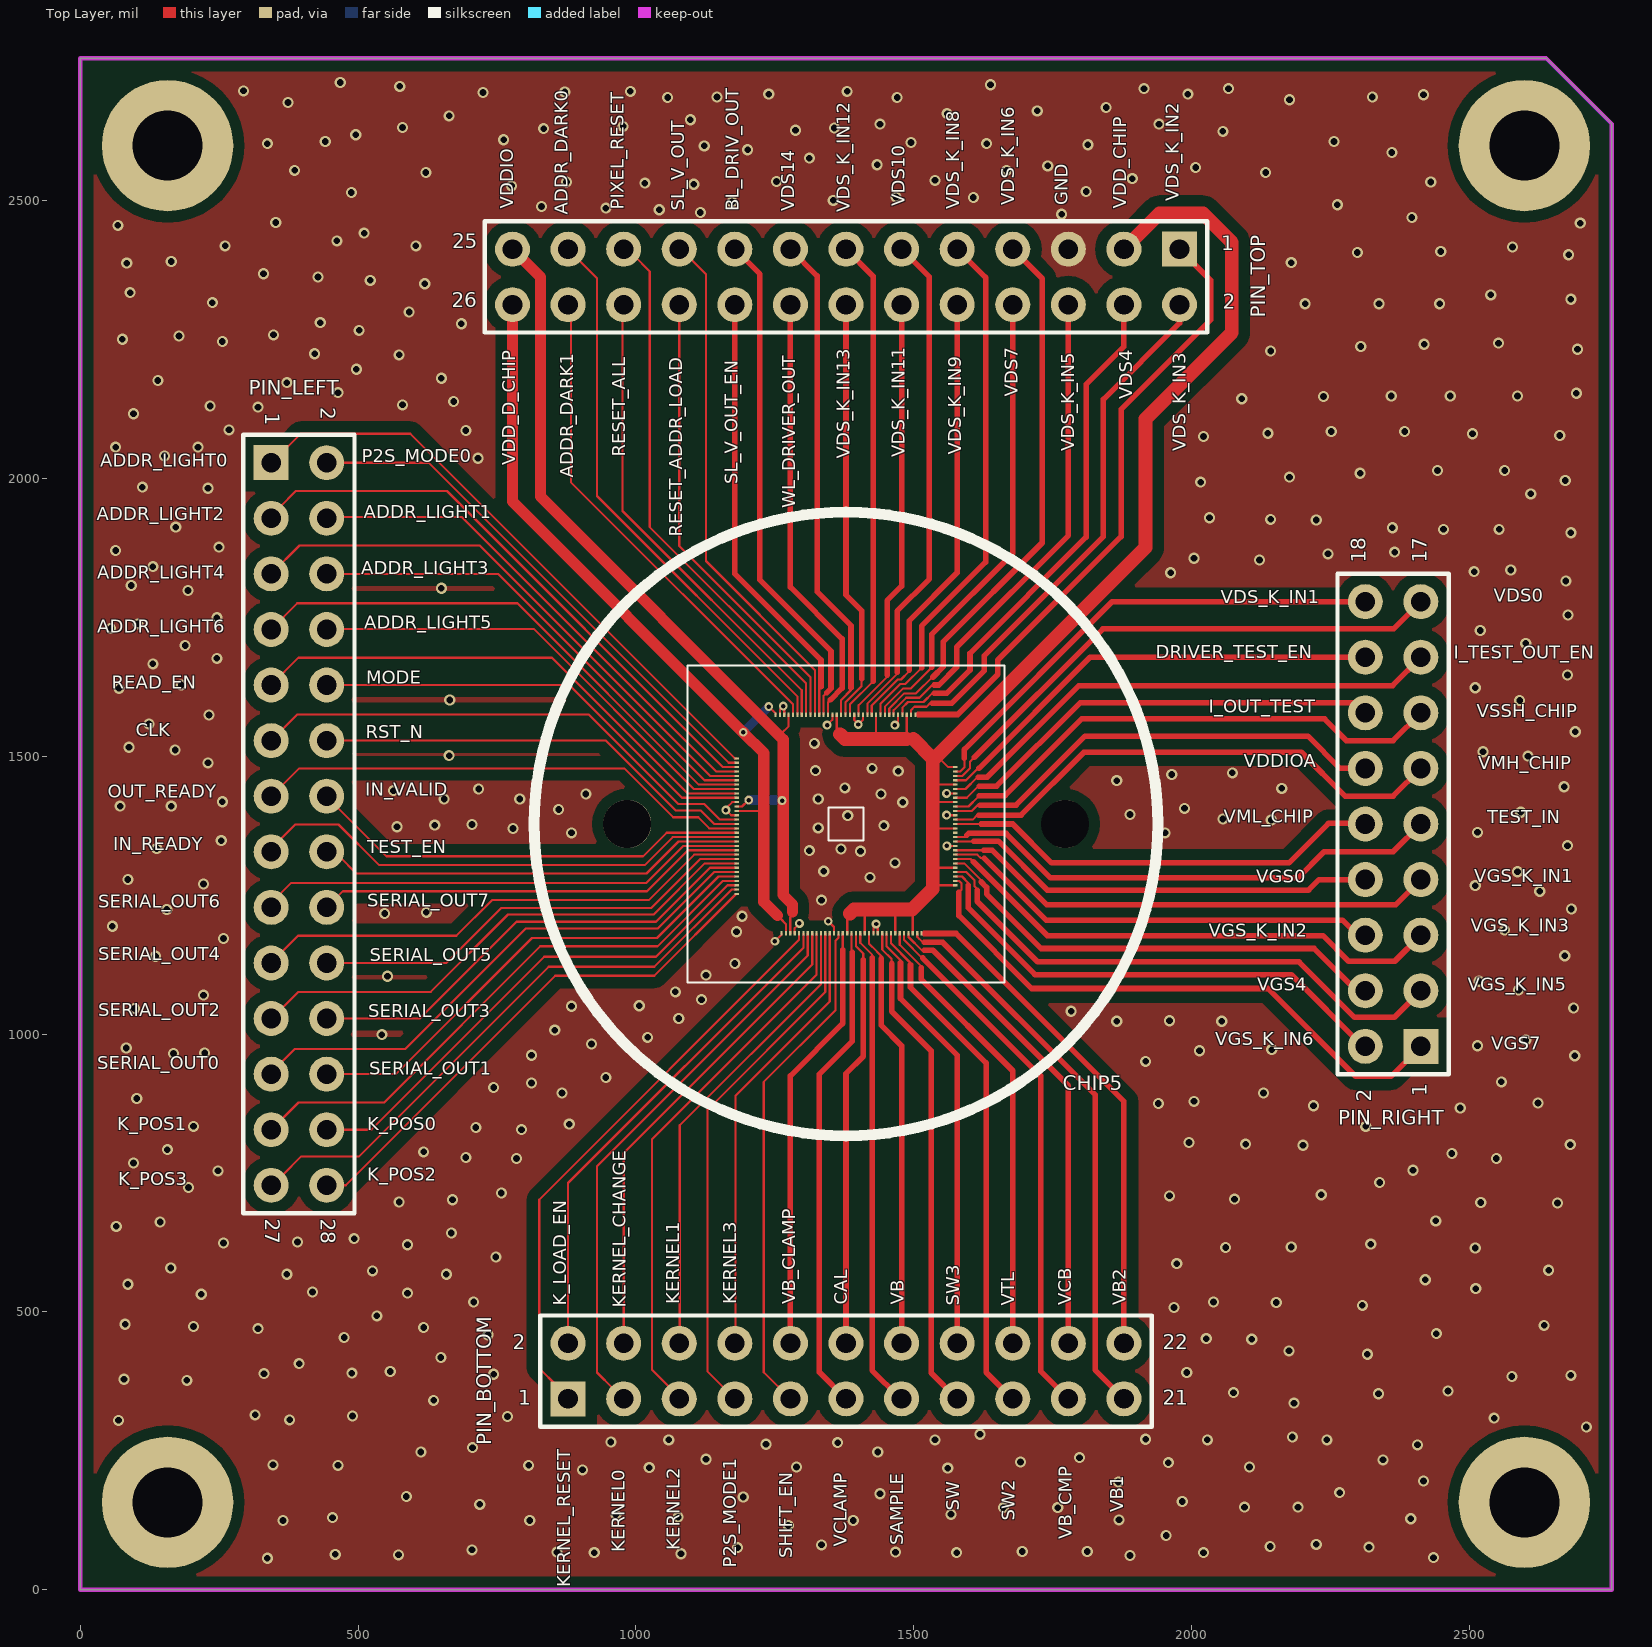
[diagram p0: Top Layer view]
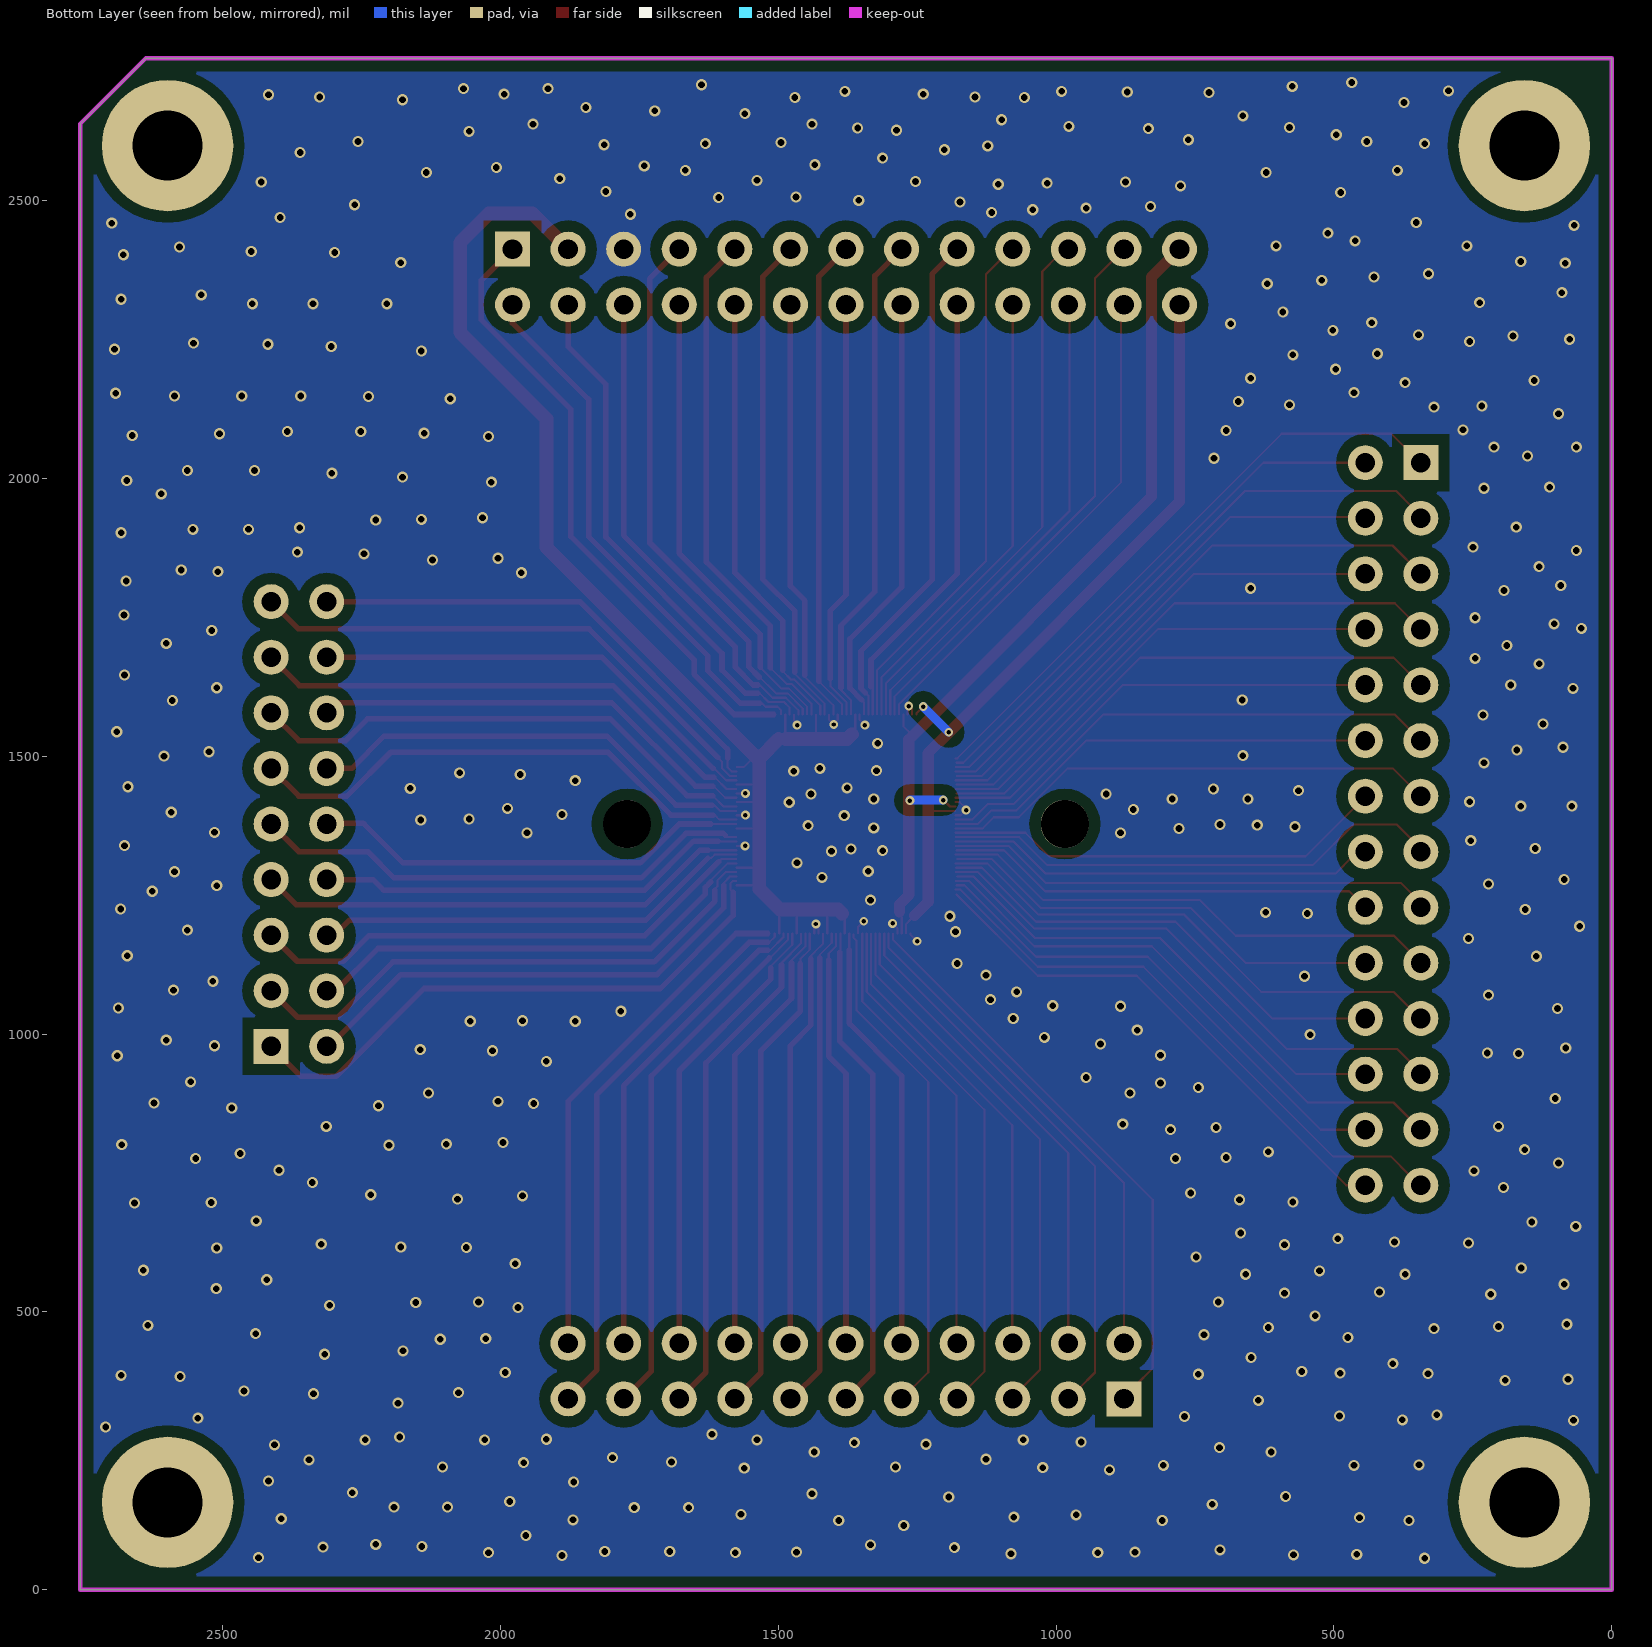
[diagram p1: Bottom Layer view, seen from below]
# Altium PCB MISC82784.pcbdoc
Units mil, origin at the board's own origin, x right, y up, seen from the top; angles counter-clockwise.
Board outline 2755.91 x 2755.91 mil, 2 copper layers (Top Layer, Bottom Layer); 5 components, 95 nets, 226 pads, 480 vias.

## Layer stack, top to bottom (the 12.6 mil dielectric is the usual default, probably not edited)
Top Layer: signal copper 1.4
Dielectric: dielectric 12.6, FR-4, Dk 4.8
Bottom Layer: signal copper 1.4

## Board outline
0,0 2755.91,0 2755.91,2637.4 2637.4,2755.91 0,2755.91

## Design rules (kind name [scope] priority, off if disabled: settings)
Clearance Clearance_2 [INPOLYGON] p1: gap=20
Clearance Clearance_1 [ispad vs ispad] p2: gap=3.9
Clearance [All] p3: gap=3.95
HoleSize [All] p1: absolutevalues=TRUE maxlimit=500 minlimit=1 maxpercent=80.000 minpercent=20.000
HoleToHoleClearance [All] p1: gap=0 allowstackedmicrovias=TRUE
MinimumSolderMaskSliver [All] p1: minsoldermaskwidth=0
PlaneConnect [All] p1: planeconnectstyle=Direct reliefexpansion=20 reliefentries=4 reliefconductorwidth=10 reliefairgap=10
PolygonConnect [All] p1: connectstyle=Direct reliefconductorwidth=10 reliefentries=4 polygonreliefangle="90 Angle"
RoutingVias [All] p1: holewidth=8 width=16 viastyle="Through Hole" minholewidth=8 minwidth=16 maxholewidth=12 maxwidth=20
SilkToSilkClearance [All] p1: silktosilkclearance=0
SilkscreenOverComponentPads [All] p1: minsilkscreentomaskgap=0
SolderMaskExpansion [All] p1: expansion=4
Width [All] p1: maxlimit=40 minlimit=3.9 preferedwidth=4 minimp=50.000000 maximp=50.000000 favimp=50.000000
22 further rules are at their usual default settings.

## Components (designator, comment, footprint, x,y, rotation, side; value= is the part's Value field where it differs from the comment)
CHIP5 "chip5" JSZ 1377.95,1377.95 r0 top locked
PIN_BOTTOM "#NAME?" HDR2.54-LI-2X11P 1377.95,393.7 r0 top
PIN_LEFT "#NAME?" HDR2.54-LI-2X14P 393.7,1377.95 r270 top
PIN_RIGHT "#NAME?" HDR2.54-LI-2X9P 2362.2,1377.95 r90 top
PIN_TOP "#NAME?" HDR2.54-LI-2X13P 1377.95,2362.2 r180 top

## Footprints (in the part's own frame and the unit in brackets; to place one, negate y for a bottom-side part, rotate by r counter-clockwise, add the part's x,y. Pads: shape width x height; smd on the part's side, far side on the other; paste and mask are expansions set on the pad)
HDR2.54-LI-2X9P [mm]
  rect 1.6x1.6 hole 0.9: 1(-10.16,-1.27)
  round 1.6 hole 0.9: 2(-10.16,1.27) 3(-7.62,-1.27) 4(-7.62,1.27) 5(-5.08,-1.27) 6(-5.08,1.27) 7(-2.54,-1.27) 8(-2.54,1.27) 9(0,-1.27) 10(0,1.27) 11(2.54,-1.27) 12(2.54,1.27) 13(5.08,-1.27) 14(5.08,1.27) 15(7.62,-1.27) 16(7.62,1.27) 17(10.16,-1.27) 18(10.16,1.27)
  silkscreen extent -11.43,-2.54 11.43,2.54
HDR2.54-LI-2X11P [mm]
  rect 1.6x1.6 hole 0.9: 1(-12.7,-1.27)
  round 1.6 hole 0.9: 2(-12.7,1.27) 3(-10.16,-1.27) 4(-10.16,1.27) 5(-7.62,-1.27) 6(-7.62,1.27) 7(-5.08,-1.27) 8(-5.08,1.27) 9(-2.54,-1.27) 10(-2.54,1.27) 11(0,-1.27) 12(0,1.27) 13(2.54,-1.27) 14(2.54,1.27) 15(5.08,-1.27) 16(5.08,1.27) 17(7.62,-1.27) 18(7.62,1.27) 19(10.16,-1.27) 20(10.16,1.27) 21(12.7,-1.27) 22(12.7,1.27)
  silkscreen extent -13.97,-2.54 13.97,2.54
HDR2.54-LI-2X13P [mm]
  rect 1.6x1.6 hole 0.9: 1(-15.24,-1.27)
  round 1.6 hole 0.9: 2(-15.24,1.27) 3(-12.7,-1.27) 4(-12.7,1.27) 5(-10.16,-1.27) 6(-10.16,1.27) 7(-7.62,-1.27) 8(-7.62,1.27) 9(-5.08,-1.27) 10(-5.08,1.27) 11(-2.54,-1.27) 12(-2.54,1.27) 13(0,-1.27) 14(0,1.27) 15(2.54,-1.27) 16(2.54,1.27) 17(5.08,-1.27) 18(5.08,1.27) 19(7.62,-1.27) 20(7.62,1.27) 21(10.16,-1.27) 22(10.16,1.27) 23(12.7,-1.27) 24(12.7,1.27) 25(15.24,-1.27) 26(15.24,1.27)
  silkscreen extent -16.51,-2.54 16.51,2.54
HDR2.54-LI-2X14P [mm]
  rect 1.6x1.6 hole 0.9: 1(-16.51,-1.27)
  round 1.6 hole 0.9: 2(-16.51,1.27) 3(-13.97,-1.27) 4(-13.97,1.27) 5(-11.43,-1.27) 6(-11.43,1.27) 7(-8.89,-1.27) 8(-8.89,1.27) 9(-6.35,-1.27) 10(-6.35,1.27) 11(-3.81,-1.27) 12(-3.81,1.27) 13(-1.27,-1.27) 14(-1.27,1.27) 15(1.27,-1.27) 16(1.27,1.27) 17(3.81,-1.27) 18(3.81,1.27) 19(6.35,-1.27) 20(6.35,1.27) 21(8.89,-1.27) 22(8.89,1.27) 23(11.43,-1.27) 24(11.43,1.27) 25(13.97,-1.27) 26(13.97,1.27) 27(16.51,-1.27) 28(16.51,1.27)
  silkscreen extent -17.78,-2.54 17.78,2.54
JSZ [mm]
  round 2.2 hole 2.2 unplated: 0(-10,0)
  oval 2x2.2 hole 2.2 unplated: 0(10,0)
  rect 0.1x0.2 smd: 1(3.177,5) 2(2.977,5) 3(2.777,5) 4(2.577,5) 5(2.377,5) 6(2.177,5) 7(1.977,5) 8(1.777,5) 9(1.577,5) 10(1.377,5) 11(1.177,5) 12(0.977,5) 13(0.777,5) 14(0.577,5) 15(0.377,5) 16(0.177,5) 17(-0.023,5) 18(-0.223,5) 19(-0.423,5) 20(-0.623,5) 21(-0.823,5) 22(-1.023,5) 23(-1.223,5) 24(-1.423,5) 25(-1.623,5) 26(-1.823,5) 27(-2.023,5) 28(-2.223,5) 29(-2.423,5) 30(-2.623,5) 31(-2.823,5) 32(-3.023,5) 33(-3.223,5) 66(-2.946,-5) 67(-2.746,-5) 68(-2.546,-5) 69(-2.346,-5) 70(-2.146,-5) 71(-1.946,-5) 72(-1.746,-5) 73(-1.546,-5) 74(-1.346,-5) 75(-1.146,-5) 76(-0.946,-5) 77(-0.746,-5) 78(-0.546,-5) 79(-0.346,-5) 80(-0.146,-5) 81(0.054,-5) 82(0.254,-5) 83(0.454,-5) 84(0.654,-5) 85(0.854,-5) 86(1.054,-5) 87(1.254,-5) 88(1.454,-5) 89(1.654,-5) 90(1.854,-5) 91(2.054,-5) 92(2.254,-5) 93(2.454,-5) 94(2.654,-5) 95(2.854,-5) 96(3.054,-5) 97(3.254,-5) 98(3.454,-5)
  rect 0.2x0.1 smd: 34(-5,3) 35(-5,2.8) 36(-5,2.6) 37(-5,2.4) 38(-5,2.2) 39(-5,2) 40(-5,1.8) 41(-5,1.6) 42(-5,1.4) 43(-5,1.2) 44(-5,1) 45(-5,0.8) 46(-5,0.6) 47(-5,0.4) 48(-5,0.2) 49(-5,0) 50(-5,-0.2) 51(-5,-0.4) 52(-5,-0.6) 53(-5,-0.8) 54(-5,-1) 55(-5,-1.2) 56(-5,-1.4) 57(-5,-1.6) 58(-5,-1.8) 59(-5,-2) 60(-5,-2.2) 61(-5,-2.4) 62(-5,-2.6) 63(-5,-2.8) 64(-5,-3) 65(-5,-3.2) 99(5,-2.8) 100(5,-2.6) 101(5,-2.4) 102(5,-2.2) 103(5,-2) 104(5,-1.8) 105(5,-1.6) 106(5,-1.4) 107(5,-1.2) 108(5,-1) 109(5,-0.8) 110(5,-0.6) 111(5,-0.4) 112(5,-0.2) 113(5,0) 114(5,0.2) 115(5,0.4) 116(5,0.6) 117(5,0.8) 118(5,1) 119(5,1.2) 120(5,1.4) 121(5,1.6) 122(5,1.8) 123(5,2) 124(5,2.2) 125(5,2.4) 126(5,2.6)
  silkscreen extent -14.25,-14.25 14.25,14.25

## Part data
PIN_BOTTOM: library part PZ254-2-11-Z-8.5
PIN_LEFT: library part PZ254-2-14-Z-8.5
PIN_RIGHT: library part PZ254-2-09-Z-8.5
PIN_TOP: library part PZ254-2-13-Z-2.5-G1

## Free pads (board coordinates)
  round 236.22 hole 125.98: 0(157.48,157.48) 0(157.48,2598.43) 0(2598.43,157.48) 0(2598.43,2598.43)

## Via types
v1: diameter 20, hole 12, Top Layer to Bottom Layer, 464 vias
v2: diameter 16, hole 8, Top Layer to Bottom Layer, 16 vias

## Nets (pads, with @x,y where several pads share a name; then routed paths per layer and width w, separated by ;. In a path a pad name is that pad's centre, name@x,y a point inside that pad or via, vN(x,y) a via of type N, cw(c..) or ccw(c..) an arc to the next point about the centre after c; other vN are vias at no path point)
ADDR_DARK0: CHIP5.28 PIN_TOP.23 | length 984
  Top Layer w3.9: PIN_TOP.23@895,2395 930,2360 930,1968 1290.44,1607.56 CHIP5.28
ADDR_DARK1: CHIP5.29 PIN_TOP.24 | length 897.9
  Top Layer w3.9: PIN_TOP.24@877,2297 886,2297 883,2294 883,1993 1282.56,1593.44 CHIP5.29
ADDR_LIGHT0: CHIP5.34 PIN_LEFT.1 | length 1061.3
  Top Layer w3.9: PIN_LEFT.1@372,2055 397,2080 594,2080 1177.94,1496.06 CHIP5.34
ADDR_LIGHT1: CHIP5.37 PIN_LEFT.4 | length 898.6
  Top Layer w3.9: PIN_LEFT.4@472,1930 687,1930 1144.56,1472.44 CHIP5.37
ADDR_LIGHT2: CHIP5.36 PIN_LEFT.3 | length 1039.8
  Top Layer w3.9: PIN_LEFT.3@359,1948 388,1977 660,1977 1156.69,1480.31 CHIP5.36
ADDR_LIGHT3: CHIP5.39 PIN_LEFT.6 | length 878.9
  Top Layer w3.9: PIN_LEFT.6@456,1828 752,1828 1123.31,1456.69 CHIP5.39
ADDR_LIGHT4: CHIP5.38 PIN_LEFT.5 | length 1028.1
  Top Layer w3.9: PIN_LEFT.5 394.75,1879 719,1879 1133.43,1464.57 CHIP5.38@1179,1464.57
ADDR_LIGHT5: CHIP5.41 PIN_LEFT.8 | length 839.4
  Top Layer w3.9: PIN_LEFT.8@461,1729 816,1729 1104.06,1440.94 CHIP5.41
ADDR_LIGHT6: CHIP5.40 PIN_LEFT.7 | length 989.9
  Top Layer w3.9: PIN_LEFT.7 390.75,1775 787,1775 1113.18,1448.82 CHIP5.40@1179,1448.82
AOUT1: CHIP5.111
BL_DRIVER_OUT: CHIP5.22 PIN_TOP.17 | length 913.2
  Top Layer w3.9: CHIP5.22 1337.68,1608.68 1342,1613
  Top Layer w10: PIN_TOP.17 1223,2367.16 1223,1817 1351,1689 1351,1622 1343,1614
CAL: CHIP5.83 PIN_BOTTOM.12 | length 755.7
  Top Layer w3.9: CHIP5.83 1395.83,1158.17 1409,1145 1409,1134
  Top Layer w10: PIN_BOTTOM.12 1377.95,928.95 1409,960 1409,1134
CLK: CHIP5.48 PIN_LEFT.11 | length 935.2
  Top Layer w3.9: PIN_LEFT.11 390.75,1575 915,1575 1076,1414 1123,1414 1151.17,1385.83 CHIP5.48
DRIVER_TEST_EN: CHIP5.123 PIN_RIGHT.16 | length 825.6
  Top Layer w3.9: CHIP5.123 1593.69,1456.69 1614,1477
  Top Layer w10: 1617,1478 1816.95,1677.95 1886,1677.95 PIN_RIGHT.16
GND: CHIP5.5 CHIP5.13 CHIP5.15 CHIP5.20 CHIP5.31 CHIP5.32 CHIP5.44 CHIP5.47 CHIP5.66 CHIP5.69 CHIP5.78 CHIP5.87 CHIP5.88 CHIP5.108 CHIP5.115 CHIP5.120 PIN_TOP.5 | length 299.4
  Top Layer w3.9: v2(1162,1403) 1171.3,1393.7 CHIP5.47 ; v2@1163,1407 1173.32,1417.32 CHIP5.44 ; v2(1250,1167) 1261.97,1178.97 CHIP5.66 ; CHIP5.32 1258.94,1583.94 v2(1265,1590) ; CHIP5.31 v2@1266.82,1585.82 ; CHIP5.69 1285.59,1190.59 v2(1294,1199) ; v2(1344,1556) 1353.43,1565.43 CHIP5.20 ; v2(1346,1203) 1356.46,1192.54 CHIP5.78 ; CHIP5.15 1392.8,1565.2 v2@1398,1560 ; v2(1400,1557) 1408.55,1565.55 CHIP5.13 ; CHIP5.87 1427.32,1193.32 v2(1432,1198) ; CHIP5.88 v2@1435.2,1190.8 ; v2(1466,1556) 1471.54,1561.54 CHIP5.5 ; v2(1559,1394) 1559.3,1393.7 CHIP5.115 ; v2(1559.07,1433.07) CHIP5.120 ; v2(1559.42,1338.58) CHIP5.108
  Bottom Layer w3.9: v2@1249,1167 v2(1250,1167)
  other v1: 337,57 2435,58 1889,62 573,63 459,64 1081,65 925,67 1577,67 2021,67 858,68 1467,68 1695,69 1812,69 705,72 1183,76 2319,77 2141,78 1334,81 2224,82 1954,98 1274,116 365,125 809,125 1391,125 1869,126 2394,128 454,130 1076,131 964,135 1567,136 1661,148 1759,148 2095,149 2191,149 719,154 1983,159 1193,167 587,168 1439,173 2266,175 1868,194 2417,196 904,216 1561,219 1024,220 1289,221 2104,221 464,224 807,224 347,225 1958,229 1692,230 2344,234 1126,235 1798,238 613,248 1435,248 706,256 2406,261 1234,262 1363,265 955,266 1059,270 1538,270 2028,270 2243,270 1917,271 2181,275 1619,280 2710,293 69,305 377,306 2544,309 769,312 490,313 315,315 2184,336 636,341 2336,353 2075,355 2461,358 192,377 79,379 2576,384 2682,386 744,388 331,389 489,390 1991,391 558,393 394,407 649,418 2316,424 2175,430 2108,451 2026,452 475,454 734,459 2440,461 320,470 618,472 204,474 2634,476 81,478 534,493 1968,508 2307,512 2152,517 708,518 2039,518 218,532 589,534 418,536 2511,542 86,550 2420,558 372,568 659,568 526,574 2642,575 163,579 1973,587 748,599 2510,615 2061,616 2179,617 589,621 2322,622 258,624 391,626 493,632 668,642 65,654 144,662 2439,664 2658,696 2520,697 574,698 670,702 2077,703 1960,709 2233,711 758,714 195,724 2338,733 248,754 2398,755 96,768 785,776 2548,776 694,778 2468,785 618,788 157,792 2200,800 2681,801 2097,802 1995,805 794,828 712,832 204,834 2313,834 880,838 2483,867 2219,871 1940,875 2623,876 2004,879 102,884 867,894 2129,894 744,904 812,912 2557,914 946,922 1917,951 2689,961 812,962 168,965 224,966 2014,970 2144,972 83,975 2514,979 920,982 2601,989 1021,994 543,999 854,1007 1865,1023 2054,1023 1960,1024 1077,1028 1783,1041 98,1046 2687,1047 884,1050 1006,1051 1118,1062 222,1070 1071,1076 2588,1079 2517,1095 553,1104 1126,1106 1178,1127 136,1140 2671,1141 258,1172 1181,1184 2563,1187 58,1194 1191,1212 548,1217 623,1219 156,1224 2683,1225 1334,1241 2626,1257 2510,1267 222,1270 86,1278 1421,1282 2586,1292 1338,1293 1466,1308 1404,1329 1312,1330 1369,1333 138,1334 2676,1339 254,1348 884,1362 1952,1362 2514,1363 779,1370 1328,1371 570,1373 1446,1375 638,1376 705,1377 2143,1385 2056,1387 1381,1393 1889,1395 2592,1399 861,1404 1987,1406 72,1410 164,1410 1480,1417 256,1418 655,1423 791,1423 1328,1423 910,1432 1441,1432 564,1438 717,1441 2162,1442 1376,1443 2670,1445 1865,1456 1964,1467 2073,1470 1472,1473 1323,1474 1425,1478 230,1488 2605,1500 664,1501 2524,1508 171,1511 88,1516 1321,1523 2690,1544 124,1558 232,1574 2590,1600 665,1601 70,1622 2510,1623 182,1628 2676,1646 131,1666 246,1676 189,1699 2601,1703 2519,1726 55,1730 104,1738 246,1749 2677,1754 194,1798 650,1802 92,1807 2673,1815 1962,1830 2508,1832 2574,1835 131,1841 2122,1853 2004,1856 2245,1864 2365,1867 64,1870 250,1876 2682,1902 2453,1908 2553,1908 2361,1911 172,1912 2224,1925 2142,1926 2032,1929 2610,1972 230,1982 112,1984 2016,1993 2672,1996 2176,2002 2303,2009 2442,2014 2563,2014 716,2036 152,2040 64,2056 212,2056 2021,2075 2662,2077 2505,2080 2137,2081 2251,2084 2383,2084 694,2086 268,2087 96,2116 320,2128 234,2130 580,2132 672,2138 2090,2143 2237,2147 2359,2148 2465,2148 2586,2148 2692,2153 464,2154 372,2172 140,2176 650,2180 497,2196 574,2222 422,2224 2142,2229 2694,2232 2304,2237 2418,2241 2552,2243 256,2246 76,2250 178,2256 348,2258 502,2266 686,2278 432,2280 592,2299 2204,2314 2337,2314 2446,2314 238,2316 2682,2322 2538,2330 90,2334 620,2350 522,2356 428,2362 330,2368 84,2387 2179,2388 164,2390 2678,2402 2298,2406 2448,2408 2577,2416 261,2418 604,2418 462,2427 511,2441 68,2455 2699,2459 352,2460 2396,2469 1766,2475 1116,2478 1042,2483 946,2486 830,2489 2262,2492 1173,2497 1355,2500 1607,2505 1468,2506 488,2514 1810,2516 776,2526 1104,2529 1016,2531 875,2533 2430,2533 1253,2534 1538,2536 1893,2539 622,2550 2133,2550 386,2554 1667,2554 2007,2559 1741,2562 1434,2564 1312,2576 2360,2586 1201,2591 1123,2598 1813,2600 337,2602 1631,2602 1495,2604 441,2606 2256,2606 762,2609 496,2618 2056,2624 1287,2626 834,2629 1357,2630 580,2631 977,2633 1439,2637 1941,2637 1098,2645 664,2652 1560,2656 1722,2661 1846,2667 374,2676 2176,2681 1057,2685 1470,2685 1146,2686 2325,2686 2417,2690 1239,2691 1993,2691 725,2694 872,2695 990,2696 1380,2696 294,2697 1914,2701 2066,2701 575,2705 1638,2708 468,2712
I_OUT_TEST: CHIP5.119 PIN_RIGHT.14 | length 813.6
  Top Layer w3.9: CHIP5.119 1595.2,1425.2 1616,1446
  Top Layer w10: 1618,1446 1649,1446 1799,1596 2294.16,1596 PIN_RIGHT.14
I_TEST_OUT_EN: CHIP5.121 PIN_RIGHT.15 | length 932.2
  Top Layer w3.9: CHIP5.121 1592.94,1440.94 1613,1461
  Top Layer w10: 1616,1462 1632,1462 1797,1627 1810,1627 2361.25,1627 PIN_RIGHT.15
IN_READY: CHIP5.52 PIN_LEFT.15 | length 901.8
  Top Layer w3.9: PIN_LEFT.15@347,1337 387,1377 465,1377 538,1304 1016,1304 1066.33,1354.33 CHIP5.52
IN_VALID: CHIP5.51 PIN_LEFT.14 | length 789
  Top Layer w3.9: PIN_LEFT.14@451,1420 551,1320 1013,1320 1055.2,1362.2 CHIP5.51
K_LOAD_EN: CHIP5.71 PIN_BOTTOM.2 | length 912.8
  Top Layer w3.9: PIN_BOTTOM.2 877.95,731.95 1301.34,1155.34 CHIP5.71
K_POS0: CHIP5.63 PIN_LEFT.26 | length 917.5
  Top Layer w3.9: PIN_LEFT.26 523.95,827.95 835,1139 1036,1139 1164.71,1267.71 CHIP5.63@1179,1267.71
K_POS1: CHIP5.62 PIN_LEFT.25 | length 1004.1
  Top Layer w3.9: PIN_LEFT.25@357,841 393,877 547,877 828,1158 1039,1158 1156.59,1275.59 CHIP5.62
K_POS2: CHIP5.65 PIN_LEFT.28 | length 952
  Top Layer w3.9: PIN_LEFT.28 477.95,727.95 855,1105 1033,1105 CHIP5.65@1179,1251
K_POS3: CHIP5.64 PIN_LEFT.27 | length 1029.9
  Top Layer w3.9: PIN_LEFT.27@364,746 398,780 502,780 843,1121 1033,1121 1171.84,1259.84 CHIP5.64
KERNEL0: CHIP5.72 PIN_BOTTOM.3 | length 988.2
  Top Layer w3.9: PIN_BOTTOM.3@959,362 930,391 930,762 1309.21,1141.21 CHIP5.72
KERNEL1: CHIP5.75 PIN_BOTTOM.6 | length 827.2
  Top Layer w3.9: PIN_BOTTOM.6@1079,459 1079,836 1332.83,1089.83 CHIP5.75
KERNEL2: CHIP5.74 PIN_BOTTOM.5 | length 962.8
  Top Layer w3.9: PIN_BOTTOM.5@1068,357 1029,396 1029,811 1324.96,1106.96 CHIP5.74
KERNEL3: CHIP5.77 PIN_BOTTOM.8 | length 789.3
  Top Layer w3.9: PIN_BOTTOM.8@1179,462 1179,889 1348.58,1058.58 CHIP5.77
KERNEL_CHANGE: CHIP5.73 PIN_BOTTOM.4 | length 877.9
  Top Layer w3.9: PIN_BOTTOM.4 977.95,785.95 1317.09,1125.09 CHIP5.73
KERNEL_RESET: CHIP5.70 PIN_BOTTOM.1 | length 1021
  Top Layer w3.9: PIN_BOTTOM.1@858,367 826,399 826,702 1293.46,1169.46 CHIP5.70
MODE: CHIP5.43 PIN_LEFT.10 | length 809.1
  Top Layer w3.9: PIN_LEFT.10@456,1628 880,1628 1082.8,1425.2 CHIP5.43
OUT_READY: CHIP5.50 PIN_LEFT.13 | length 879.9
  Top Layer w3.9: PIN_LEFT.13@360,1444 394,1478 979,1478 1067,1390 1112,1390 1131.92,1370.08 CHIP5.50
P2S_MODE0: CHIP5.35 PIN_LEFT.2 | length 958.9
  Top Layer w3.9: PIN_LEFT.2 627.05,2027.95 1166.81,1488.19 CHIP5.35@1179,1488.19
P2S_MODE1: CHIP5.76 PIN_BOTTOM.7 | length 945.4
  Top Layer w3.9: PIN_BOTTOM.7 1129,392.65 1129,864 1340.71,1075.71 CHIP5.76
PIXEL_RESET_EN: CHIP5.26 PIN_TOP.21 | length 956.1
  Top Layer w3.9: PIN_TOP.21@995,2402 1025,2372 1025,1912 1306.19,1630.81 CHIP5.26
READ_EN: CHIP5.42 PIN_LEFT.9 | length 956.7
  Top Layer w3.9: PIN_LEFT.9 392.75,1677 849,1677 1092.92,1433.08 CHIP5.42@1179,1433.08
RESET_ADDR_LOAD: CHIP5.25 PIN_TOP.20 | length 835.2
  Top Layer w3.9: PIN_TOP.20@1077.95,2311 PIN_TOP.20 ; PIN_TOP.20@1078,2311 1078,1878 1314.06,1641.94 CHIP5.25
RESET_ALL: CHIP5.27 PIN_TOP.22 | length 870.9
  Top Layer w3.9: PIN_TOP.22@976,2301 976,1941 1298.31,1618.69 CHIP5.27 ; PIN_TOP.22@977.95,2301 PIN_TOP.22
RST_N: CHIP5.49 PIN_LEFT.12 | length 799.5
  Top Layer w3.9: PIN_LEFT.12 946.05,1527.95 1072,1402 1117,1402 1141.05,1377.95 CHIP5.49
SAMPLE: CHIP5.84 PIN_BOTTOM.13 | length 868.6
  Top Layer w3.9: CHIP5.84 1403.7,1164.3 1425,1143 1425,1137
  Top Layer w10: 1425,1137 1425,395 PIN_BOTTOM.13@1473,347 ; PIN_BOTTOM.13@1473.83,347.83 PIN_BOTTOM.13
SERIAL_OUT0: CHIP5.60 PIN_LEFT.23 | length 966.6
  Top Layer w3.9: PIN_LEFT.23@358,945 386,973 585,973 802,1190 1039,1190 1140.34,1291.34 CHIP5.60
SERIAL_OUT1: CHIP5.61 PIN_LEFT.24 | length 881.6
  Top Layer w3.9: PIN_LEFT.24 567.95,927.95 813,1173 1038,1173 1148.47,1283.47 CHIP5.61@1178,1283.47
SERIAL_OUT2: CHIP5.58 PIN_LEFT.21 | length 934.7
  Top Layer w3.9: PIN_LEFT.21@357,1040 393,1076 631,1076 770,1215 1032,1215 1124.09,1307.09 CHIP5.58
SERIAL_OUT3: CHIP5.59 PIN_LEFT.22 | length 848.7
  Top Layer w3.9: PIN_LEFT.22 610.95,1027.95 785,1202 1036,1202 1133.21,1299.21 CHIP5.59@1180,1299.21
SERIAL_OUT4: CHIP5.56 PIN_LEFT.19 | length 894.8
  Top Layer w3.9: PIN_LEFT.19@360,1145 392,1177 677,1177 741,1241 1023,1241 1104.83,1322.83 CHIP5.56
SERIAL_OUT5: CHIP5.57 PIN_LEFT.20 | length 811.8
  Top Layer w3.9: PIN_LEFT.20 658.95,1127.95 758,1227 1028,1227 1115.97,1314.97 CHIP5.57@1178,1314.97
SERIAL_OUT6: CHIP5.54 PIN_LEFT.17 | length 865.5
  Top Layer w3.9: PIN_LEFT.17@354,1246 380,1272 1019,1272 1085.58,1338.58 CHIP5.54
SERIAL_OUT7: CHIP5.55 PIN_LEFT.18 | length 777.9
  Top Layer w3.9: PIN_LEFT.18 472.75,1257 1020,1257 1093.71,1330.71 CHIP5.55@1179,1330.71
SHIFT_EN: CHIP5.79 PIN_BOTTOM.9 | length 910.8
  Top Layer w3.9: PIN_BOTTOM.9 1230,391.65 1230,914 1359,1043 1359,1168 1364.34,1173.34 CHIP5.79@1364.34,1179
SL_V_OUT: CHIP5.24 PIN_TOP.19 | length 918.6
  Top Layer w3.9: PIN_TOP.19@1094,2399 1126,2367 1126,1851 1321.94,1655.06 CHIP5.24
SL_V_OUT_EN: CHIP5.23 PIN_TOP.18 | length 803
  Top Layer w3.9: CHIP5.23 1329.81,1621.81 1333,1625
  Top Layer w10: PIN_TOP.18 1177.95,1828.05 1333,1673 1333,1625.16 1332.84,1625
SW: CHIP5.89 PIN_BOTTOM.15 | length 893.3
  Top Layer w3.9: CHIP5.89 1443.07,1151.93 1460,1135 1460,1127
  Top Layer w10: 1460,1127 1460,1041 1531,970 1531,390.65 PIN_BOTTOM.15
SW2: CHIP5.91 PIN_BOTTOM.17 | length 928.2
  Top Layer w3.9: CHIP5.91 1458.82,1163.18 1494,1128 1494,1125
  Top Layer w10: 1494,1125 1494,1084 1630,948 1630,391.65 PIN_BOTTOM.17
SW3: CHIP5.90 PIN_BOTTOM.16 | length 790.4
  Top Layer w3.9: CHIP5.90 1450.94,1168 1450.94,1166.06 1450.94,1158.06 1477,1132 1477,1128
  Top Layer w10: 1476,1128 1476,1064 1577.95,962.05 PIN_BOTTOM.16
TEST_EN: CHIP5.53 PIN_LEFT.16 | length 751.7
  Top Layer w3.9: PIN_LEFT.16@466,1320 497,1289 1019,1289 1076.46,1346.46 CHIP5.53
TEST_IN: CHIP5.110 PIN_RIGHT.9 | length 913.9
  Top Layer w3.9: CHIP5.110 1593.33,1354.33 1595.68,1356.68
  Top Layer w10: 1595,1357.36 1598.64,1361 1608,1361 1666,1361 1746,1281 2191,1281 2238,1328 2362.25,1328 PIN_RIGHT.9
VB: CHIP5.86 PIN_BOTTOM.14 | length 761.6
  Top Layer w3.9: CHIP5.86 1419.45,1162.55 1434,1148 1436,1146 1441,1141 1441,1136
  Top Layer w10: 1441,1136 1441,1016 1477.95,979.05 PIN_BOTTOM.14
VB1: CHIP5.97 PIN_BOTTOM.21 | length 1012.7
  Top Layer w3.9: CHIP5.97 1506.06,1174.73 1509.52,1171.27 1509.73,1171.27 1516,1165 1519,1165
  Top Layer w10: 1519,1165 1552,1165 1826,891 1826,395.65 PIN_BOTTOM.21
VB2: CHIP5.98 PIN_BOTTOM.22 | length 919.4
  Top Layer w10: 1519,1181 1576,1181 1877.95,879.05 PIN_BOTTOM.22
VB_CLAMP: CHIP5.80 PIN_BOTTOM.10 | length 776.4
  Top Layer w3.9: 1372.2,1152 CHIP5.80
  Top Layer w10: PIN_BOTTOM.10 1277.95,924.95 1372,1019 1372,1152
VB_CMP: CHIP5.94 PIN_BOTTOM.19 | length 960
  Top Layer w3.9: CHIP5.94 1482.44,1169.56 1515.31,1136.69
  Top Layer w10: 1515.68,1137.05 1728,924.73 1728,393.65 PIN_BOTTOM.19
VCB: CHIP5.95 PIN_BOTTOM.20 | length 868.3
  Top Layer w3.9: CHIP5.95 1490.31,1174.69 1514,1151 1519,1151
  Top Layer w10: 1519,1151 1534,1151 1777.95,907.05 PIN_BOTTOM.20
VCLAMP: CHIP5.82 PIN_BOTTOM.11 | length 879.7
  Top Layer w3.9: 1387.95,1149.05 CHIP5.82
  Top Layer w10: PIN_BOTTOM.11 1330,391.65 1330,928 1389,987 1389,1147
VDD_CHIP: CHIP5.3 CHIP5.10 CHIP5.19 CHIP5.81 CHIP5.85 CHIP5.92 CHIP5.96 CHIP5.99 CHIP5.103 CHIP5.112 CHIP5.118 CHIP5.122 CHIP5.126 PIN_TOP.3 | length 2461.6
  Top Layer w3.9: CHIP5.19 1361.31,1548.69 1369,1541 ; CHIP5.81 1380.08,1216.08 ; CHIP5.85 1411.57,1213.57 ; 1432.17,1531 CHIP5.10 ; CHIP5.92 1466.69,1215.69 ; 1487.29,1531 CHIP5.3 ; 1491,1224 1498.19,1216.81 CHIP5.96 ; 1534,1299.21 CHIP5.103 ; 1534,1417.32 CHIP5.118 ; 1534,1448.82 CHIP5.122 ; 1536,1267.72 CHIP5.99 ; 1537,1370.08 CHIP5.112 ; 1550,1492 1561.69,1480.31 CHIP5.126
  Top Layer w25: 1367.5,1539.5 1376,1531 1432.17,1531 1487.29,1531 ; 1385,1217 1392,1224 1491,1224 ; 1497,1224 1534,1261 1534,1299.21 1534,1417.32 1534,1448.82 1534,1492 1917,1875 1917,2107 2072,2262 2072,2424 2020,2476 1941.75,2476 PIN_TOP.3 ; 1499,1531 1533,1497
VDD_D_CHIP: CHIP5.33 CHIP5.46 CHIP5.67 PIN_TOP.26 | length 1460.9
  Top Layer w3.9: CHIP5.46 1230,1401.57 1231.43,1401.57 ; v2(1239,1589) 1251.07,1576.93 CHIP5.33 ; 1261,1207 1269.84,1198.16 CHIP5.67
  Top Layer w20: PIN_TOP.26 777.95,1958.05 v2(1193,1543) 1230,1506 1230,1401.57 1230,1238 1255,1213
  Bottom Layer w16: v2(1193,1543) v2(1239,1589)
VDDIO: CHIP5.30 CHIP5.45 CHIP5.68 PIN_TOP.25 | length 1560.2
  Top Layer w3.9: CHIP5.45 1191,1409.45 v2@1202,1420.45 ; 1262,1541 1274.69,1553.69 CHIP5.30 ; CHIP5.68 1277.72,1209.72 1282,1214
  Top Layer w20: PIN_TOP.25 828,2362.16 828,1967 1265,1530 1265,1250 1282,1233 1282,1220
  Bottom Layer w16: v2(1203,1421) v2@1263,1421
  other v2: 1263,1420
VDDIOA: CHIP5.116 PIN_RIGHT.12 | length 822.1
  Top Layer w3.9: CHIP5.116 1604.57,1401.57 1615,1412 1619,1412 1624,1412
  Top Layer w10: 1619,1412 1684,1412 1808,1536 2209,1536 2267.05,1477.95 PIN_RIGHT.12
VDS0: CHIP5.124 PIN_RIGHT.17 | length 971.4
  Top Layer w3.9: CHIP5.124 1587.57,1464.57 1601,1478 1601,1490 1607,1496
  Top Layer w10: 1609,1498 1840,1729 2363.25,1729 PIN_RIGHT.17
VDS4: CHIP5.4 PIN_TOP.4 | length 936.4
  Top Layer w3.9: CHIP5.4 1479.42,1587.21 1489.5,1597.3 1502,1597.3 ; 1504,1597.3 1502,1597.3 ; 1537,1614 1534,1614 1517.3,1597.3 1502,1597.3
  Top Layer w10: 1537,1613 1559,1613 1601,1655 1601,1685 1810,1894 1810,2169 1877.95,2236.95 PIN_TOP.4
VDS7: CHIP5.8 PIN_TOP.8 | length 840.5
  Top Layer w3.9: CHIP5.8 1447.92,1589.02 1480.9,1622 1485,1622 ; 1487,1622 1485,1622 ; 1531,1658 1495,1622 1485,1622
  Top Layer w10: 1532,1660 1532,1719 1677.95,1864.95 PIN_TOP.8
VDS10: CHIP5.12 PIN_TOP.11 | length 904.3
  Top Layer w3.9: CHIP5.12 1416.42,1594.42 1470,1648 1470,1651
  Top Layer w10: 1470,1651 1470,1761 1528,1819 1528,2362.16 PIN_TOP.11
VDS14: CHIP5.18 PIN_TOP.15 | length 890
  Top Layer w3.9: CHIP5.18 1369.18,1601.18 1387,1619 1387,1623
  Top Layer w10: PIN_TOP.15 1326,2364.16 1326,1796 1387,1735 1387,1623
VDS_K_IN1: CHIP5.125 PIN_RIGHT.18 | length 882.7
  Top Layer w3.9: CHIP5.125 1583.44,1472.44 1591,1480 1591,1496
  Top Layer w10: 1591,1496 1591,1512 1856.95,1777.95 PIN_RIGHT.18
VDS_K_IN2: CHIP5.1 PIN_TOP.1 | length 1119.9
  Top Layer w10: 1508,1575 1579,1575 1651,1647 1651,1673 1873,1895 1873,2124 2034,2285 2034,2356.16 PIN_TOP.1
VDS_K_IN3: CHIP5.2 PIN_TOP.2 | length 980.1
  Top Layer w3.9: CHIP5.2 1495.16,1583.16 1501,1589 1523,1589 1529,1595 1533,1595 1540,1595
  Top Layer w10: 1533,1595 1568,1595 1627,1654 1627,1681 1841,1895 1841,2142 1977.95,2278.95 PIN_TOP.2
VDS_K_IN5: CHIP5.6 PIN_TOP.6 | length 889.6
  Top Layer w3.9: CHIP5.6 1463.67,1582.57 1486.25,1605.15 1510.15,1605.15 1533,1628 1538,1628
  Top Layer w10: 1537,1628 1538,1628 1545,1628 1577,1660 1577,1696 1777.95,1896.95 PIN_TOP.6
VDS_K_IN6: CHIP5.7 PIN_TOP.7 | length 992.7
  Top Layer w3.9: CHIP5.7 1455.79,1585.79 1483,1613 1495,1613 ; 1501,1613 1495,1613 ; 1534,1643 1504,1613 1495,1613
  Top Layer w10: 1534,1642 1553,1661 1553,1706 1731,1884 1731,2359.16 PIN_TOP.7
VDS_K_IN8: CHIP5.9 PIN_TOP.9 | length 942.1
  Top Layer w3.9: CHIP5.9 1440.05,1594.05 1476,1630 1485,1630 1514,1659
  Top Layer w10: 1514,1659 1514,1734 1629,1849 1629,2361.16 PIN_TOP.9
VDS_K_IN9: CHIP5.11 PIN_TOP.10 | length 804.1
  Top Layer w3.9: CHIP5.11 1424.3,1584.3 1424.3,1591.2 1471.1,1638 1477,1638 1491,1652 1491,1655
  Top Layer w10: 1492,1655 1492,1744 1577.95,1829.95 PIN_TOP.10
VDS_K_IN11: CHIP5.14 PIN_TOP.12 | length 769.4
  Top Layer w3.9: CHIP5.14 1400.68,1591.68 1452,1643 1452,1646
  Top Layer w10: 1452,1646 1452,1780 1477.95,1805.95 PIN_TOP.12
VDS_K_IN12: CHIP5.16 PIN_TOP.13 | length 875.1
  Top Layer w3.9: CHIP5.16 1384.93,1592.93 1427,1635
  Top Layer w10: PIN_TOP.13 1427,2363.16 1427,1635
VDS_K_IN13: CHIP5.17 PIN_TOP.14 | length 767.1
  Top Layer w3.9: CHIP5.17 1377.05,1597.05 1406,1626 1406,1639
  Top Layer w10: 1377.95,1813.95 1377.95,1820 ; PIN_TOP.14 1377.95,1820 ; 1406,1639 1406,1762 1377.95,1790.05 1377.95,1820
VGS0: CHIP5.109 PIN_RIGHT.8 | length 781.3
  Top Layer w3.9: CHIP5.109 1607.54,1346.46
  Top Layer w10: 1608,1347.05 1651.95,1347.05 1740,1259 2210,1259 2228.95,1277.95 PIN_RIGHT.8
VGS4: CHIP5.104 PIN_RIGHT.4 | length 840.5
  Top Layer w3.9: CHIP5.104 1590.91,1307.09 1622,1276 1622,1275
  Top Layer w10: 1621,1274 1631,1264 1631,1252 1729,1154 2220,1154 2296.05,1077.95 PIN_RIGHT.4
VGS7: CHIP5.100 PIN_RIGHT.1 | length 1046.3
  Top Layer w3.9: CHIP5.100 1581.18,1275.59 1586,1270.77 1586,1260 1581,1255
  Top Layer w10: 1581,1255 1581,1213 1712,1082 2137,1082 2295,924 2358.25,924 PIN_RIGHT.1
VGS_K_IN1: CHIP5.107 PIN_RIGHT.7 | length 896.6
  Top Layer w3.9: CHIP5.107 1626,1330.71
  Top Layer w10: 1626,1331 1641,1331 1739,1233 2367.25,1233 PIN_RIGHT.7
VGS_K_IN2: CHIP5.106 PIN_RIGHT.6 | length 795
  Top Layer w3.9: CHIP5.106 1614.17,1322.83 1620,1317 1625,1317
  Top Layer w10: 1627,1316 1738,1205 2271,1205 2298.05,1177.95 PIN_RIGHT.6
VGS_K_IN3: CHIP5.105 PIN_RIGHT.5 | length 933
  Top Layer w3.9: CHIP5.105 1602.04,1314.96 1607,1310
  Top Layer w10: 1607,1310 1740,1177 2236,1177 2282,1131 2365.25,1131 PIN_RIGHT.5
VGS_K_IN5: CHIP5.102 PIN_RIGHT.3 | length 986.4
  Top Layer w3.9: CHIP5.102 1594.66,1291.34 1609,1277 1609,1274 1609,1266 1615,1260 ; 1615.5,1260.5 1617,1259
  Top Layer w10: 1614,1259 1614,1239 1723,1130 2193,1130 2293,1030 2364.25,1030 PIN_RIGHT.3
VGS_K_IN6: CHIP5.101 PIN_RIGHT.2 | length 890.7
  Top Layer w3.9: CHIP5.101 1586.54,1283.46 1599,1271 1599,1268
  Top Layer w10: 1598,1268 1598,1227 1718,1107 2179,1107 2308.05,977.95 PIN_RIGHT.2
VMH_CHIP: CHIP5.114 PIN_RIGHT.11 | length 945
  Top Layer w3.9: CHIP5.114 1605.83,1385.83 1614,1394 1617,1394 1621,1394
  Top Layer w10: 1617,1394 1693,1394 1806,1507 2197,1507 2276,1428 2362.25,1428 PIN_RIGHT.11
VML_CHIP: CHIP5.113 PIN_RIGHT.10 | length 799.6
  Top Layer w3.9: CHIP5.113 1619.05,1377.95
  Top Layer w10: 1621,1378 1678,1378 1748,1308 2175,1308 2246,1379 PIN_RIGHT.10@2318,1379
VSSH_CHIP: CHIP5.117 PIN_RIGHT.13 | length 936.7
  Top Layer w3.9: CHIP5.117 1598.45,1409.45 1616,1427
  Top Layer w10: 1618,1429 1664,1429 1802,1567 2239,1567 2278,1528 2362.25,1528 PIN_RIGHT.13
VTL: CHIP5.93 PIN_BOTTOM.18 | length 820.1
  Top Layer w3.9: CHIP5.93 1474.57,1160.43 1514,1121
  Top Layer w10: 1513,1119 1513,1099 1677.95,934.05 PIN_BOTTOM.18
WL_DRIVER_OUT: CHIP5.21 PIN_TOP.16 | length 786.4
  Top Layer w3.9: CHIP5.21 1345.56,1596.56 1350,1601
  Top Layer w10: PIN_TOP.16 1277.95,1804.05 1371,1711 1371,1622.27 1349.86,1601.14
pads on no net: CHIP5.0

## Polygon pours and split planes (outlines as drawn)
GND on Bottom Layer "Bottom Layer-No Net" (solid, remove dead copper, pour order 1000): -158,2533 -139,2514 -139,-209 2856,-209 2984,-81 3016,-49 3016,-36 3016,2777 2874,2919 2797,2996 2629,2996 35,2996 -106,2855 -151,2810 -151,2578
GND on Top Layer "Bottom Layer-No Net" (solid, remove dead copper, pour order 1001): -199,2402 -199,-29 -123,-105 -24,-204 310,-204 2847,-204 2969,-82 2998,-53 2998,-52 2998,2706 2788,2916 2729,2975 2630,2975 -46,2975 -140,2881 -181,2840 -181,2419

## Keep-outs
Board Outline Layer:
  the board outline again, w7.87

## Silkscreen, mask and mechanical layers (free items; w line width, h text height)
Top Silkscreen Layer:
  text "VDS_K_IN2" at 1985,2498 h40 r90
  text "VDS_K_IN6" at 1689,2491 h40 r90
  text "GND" at 1785,2491 h40 r90
  text "VDS10" at 1492,2489 h40 r90
  text "VDDIO" at 787,2485 h40 r90
  text "VDD_CHIP" at 1890,2485 h40 r90
  text "VDS_K_IN8" at 1590,2484 h40 r90
  text "PIXEL_RESET" at 986,2483 h40 r90
  text "SL_V_OUT" at 1095,2481 h40 r90
  text "BL_DRIV_OUT" at 1193,2480 h40 r90
  text "VDS14" at 1293,2480 h40 r90
  text "VDS_K_IN12" at 1393,2479 h40 r90
  text "ADDR_DARK0" at 885,2474 h40 r90
  text "VDS7" at 1695,2147 h40 r90
  text "VDS4" at 1901,2142 h40 r90
  text "VDS_K_IN5" at 1797,2049 h40 r90
  text "VDS_K_IN3" at 1997,2049 h40 r90
  text "VDS_K_IN9" at 1593,2042 h40 r90
  text "RESET_ALL" at 989,2039 h40 r90
  text "VDS_K_IN11" at 1492,2038 h40 r90
  text "VDS_K_IN13" at 1393,2035 h40 r90
  text "VDD_D_CHIP" at 791,2023 h40 r90
  text "P2S_MODE0" at 507,2021 h40
  text "ADDR_LIGHT0" at 36,2013 h40
  text "ADDR_DARK1" at 895,2001 h40 r90
  text "SL_V_OUT_EN" at 1191,1989 h40 r90
  text "WL_DRIVER_OUT" at 1295,1946 h40 r90
  text "ADDR_LIGHT1" at 510,1920 h40
  text "ADDR_LIGHT2" at 30,1916 h40
  text "RESET_ADDR_LOAD" at 1091,1895 h40 r90
  text "ADDR_LIGHT3" at 506,1819 h40
  text "ADDR_LIGHT4" at 31,1811 h40
  text "VDS0" at 2543,1770 h40
  text "VDS_K_IN1" at 2052,1767 h40
  text "ADDR_LIGHT5" at 511,1721 h40
  text "ADDR_LIGHT6" at 31,1714 h40
  text "DRIVER_TEST_EN" at 1935,1668 h40
  text "I_TEST_OUT_EN" at 2471,1667 h40
  text "MODE" at 515,1622 h40
  text "READ_EN" at 57,1613 h40
  text "I_OUT_TEST" at 2031,1570 h40
  text "VSSH_CHIP" at 2513,1562 h40
  text "CLK" at 100,1528 h40
  text "RST_N" at 514,1524 h40
  text "VDDIOA" at 2094,1472 h40
  text "VMH_CHIP" at 2515,1468 h40
  text "IN_VALID" at 513,1421 h40
  text "OUT_READY" at 50,1417 h40
  text "VML_CHIP" at 2058,1372 h40
  text "TEST_IN" at 2532,1371 h40
  text "IN_READY" at 60,1323 h40
  text "TEST_EN" at 517,1317 h40
  text "VGS_K_IN1" at 2508,1265 h40
  text "VGS0" at 2116,1264 h40
  text "SERIAL_OUT7" at 517,1221 h40
  text "SERIAL_OUT6" at 33,1219 h40
  text "VGS_K_IN3" at 2502,1176 h40
  text "VGS_K_IN2" at 2031,1167 h40
  text "SERIAL_OUT4" at 33,1125 h40
  text "SERIAL_OUT5" at 521,1123 h40
  text "VGS4" at 2118,1070 h40
  text "VGS_K_IN5" at 2497,1070 h40
  text "SERIAL_OUT2" at 33,1024 h40
  text "SERIAL_OUT3" at 518,1022 h40
  text "VGS_K_IN6" at 2042,972 h40
  text "VGS7" at 2539,964 h40
  text "SERIAL_OUT0" at 31,929 h40
  text "SERIAL_OUT1" at 520,919 h40
  text "K_POS1" at 67,819 h40
  text "K_POS0" at 517,819 h40
  text "K_POS2" at 517,728 h40
  text "K_POS3" at 69,720 h40
  text "KERNEL1" at 1086,514 h40 r90
  text "KERNEL3" at 1189,514 h40 r90
  text "VB_CLAMP" at 1295,514 h40 r90
  text "CAL" at 1388,513 h40 r90
  text "VB" at 1490,513 h40 r90
  text "VCB" at 1791,512 h40 r90
  text "VB2" at 1889,512 h40 r90
  text "K_LOAD_EN" at 883,511 h40 r90
  text "SW3" at 1590,511 h40 r90
  text "VTL" at 1689,511 h40 r90
  text "KERNEL_CHANGE" at 990,508 h40 r90
  text "SW" at 1590,142 h40 r90
  text "VB1" at 1885,140 h40 r90
  text "SW2" at 1690,124 h40 r90
  text "VB_CMP" at 1792,91 h40 r90
  text "SAMPLE" at 1489,80 h40 r90
  text "VCLAMP" at 1387,78 h40 r90
  text "KERNEL2" at 1087,71 h40 r90
  text "KERNEL0" at 988,68 h40 r90
  text "SHIFT_EN" at 1289,57 h40 r90
  text "P2S_MODE1" at 1189,40 h40 r90
  text "KERNEL_RESET" at 890,5 h40 r90